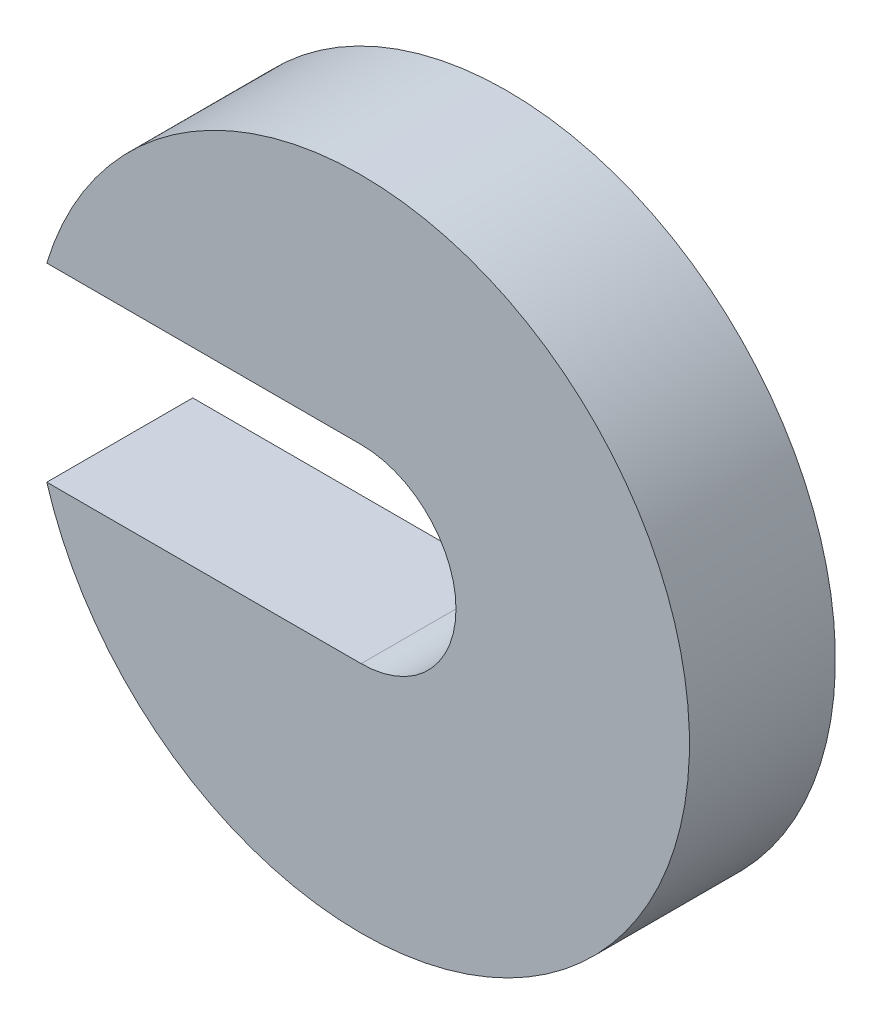
from build123d import *

# Parameters (mm, degrees)
BOSS_EXTRUDE1_DEPTH = 10


with BuildPart() as part:
    # Sketch1 → Boss-Extrude1 (new body)
    with BuildSketch(Plane.XY):
        with BuildLine():
            Line((0, 6.5), (-21.540659229, 6.5))
            ThreePointArc((-21.540659229, 6.5), (22.5, 0), (-21.540659229, -6.5))
            Line((-21.540659229, -6.5), (0, -6.5))
            ThreePointArc((0, -6.5), (6.5, 0), (0, 6.5))
        make_face()
    extrude(amount=BOSS_EXTRUDE1_DEPTH)


solid = part.part
